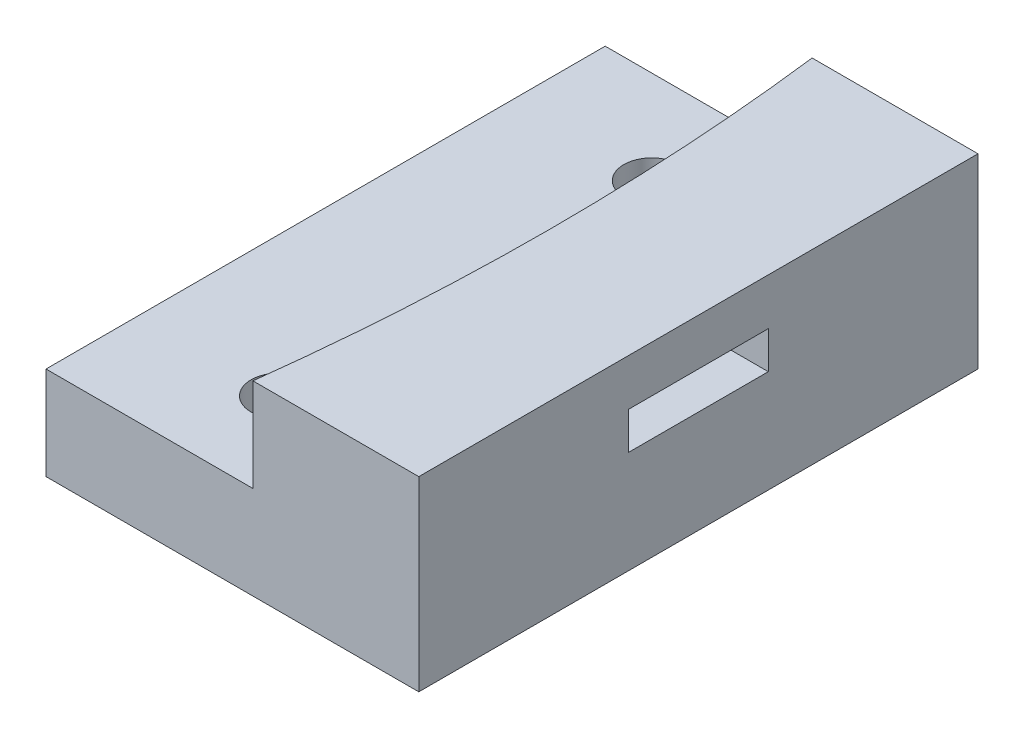
SolidWorks part; units mm, degrees
ref_plane "Front Plane" through (0, 0, 0) normal (0, 0, 1) x (1, 0, 0)
ref_plane "Top Plane" through (0, 0, 0) normal (0, 1, 0) x (1, 0, 0)
ref_plane "Right Plane" through (0, 0, 0) normal (1, 0, 0) x (0, 0, -1)
sketch "Sketch1" plane through (0, 0, 0) normal (0, 0, 1) x (1, 0, 0)
  line L0 (0, 0) -> (0, -20)
  line L1 (0, -20) -> (40, -20)
  line L2 (40, -20) -> (40, 0)
  line L5 (40, 0) -> (0, 0)
  dimension "D1" = 20
  dimension "D2" = 40
extrude "Boss-Extrude1" add sketch "Sketch1" along normal blind 60
sketch "Sketch2" plane through (0, 0, 0) normal (0, 1, 0) x (1, 0, 0)
  line L0 (40, 0) -> (0, 0) construction
  line L1 (40, -60) -> (0, -60) construction
  line L2 (22.2, 0) -> (0, 0)
  line L3 (0, 0) -> (0, -60)
  line L4 (0, -60) -> (22.2, -60)
  arc A0 (22.2, 0) -> (22.2, -60) centre (-220.9563, -30) cw
  dimension "D2" = 245
  dimension "D1" = 22.2
extrude "Cut-Extrude1" cut sketch "Sketch2" against normal blind 10
sketch "Sketch3" plane through (0, -10, 0) normal (0, 1, 0) x (1, 0, 0)
  line L0 (0, 0) -> (0, -60) construction
  line L1 (22.2, 0) -> (0, 0) construction
  circle A0 centre (15, -10) radius 3
  circle A1 centre (15, -50) radius 3
  dimension "D3" = 6
  dimension "D1" = 40
  dimension "D2" = 15
  dimension "D4" = 10
extrude "Cut-Extrude2" cut sketch "Sketch3" against normal blind 10
sketch "Sketch4" plane through (40, 0, 0) normal (1, 0, 0) x (0, 0, -1)
  line L0 (-60, -20) -> (-60, 0) construction
  line L1 (-37.5, -5) -> (-22.5, -5)
  line L2 (-37.5, -5) -> (-37.5, -9)
  line L3 (-37.5, -9) -> (-22.5, -9)
  line L4 (-22.5, -5) -> (-22.5, -9)
  line L5 (-37.5, -5) -> (-22.5, -9) construction
  line L6 (-37.5, -9) -> (-22.5, -5) construction
  line L7 (-60, -20) -> (0, -20) construction
  point P0 (-30, -7)
  dimension "D1" = 15
  dimension "D2" = 4
  dimension "D3" = 30
  dimension "D4" = 11
extrude "Cut-Extrude3" cut sketch "Sketch4" against normal blind 49
